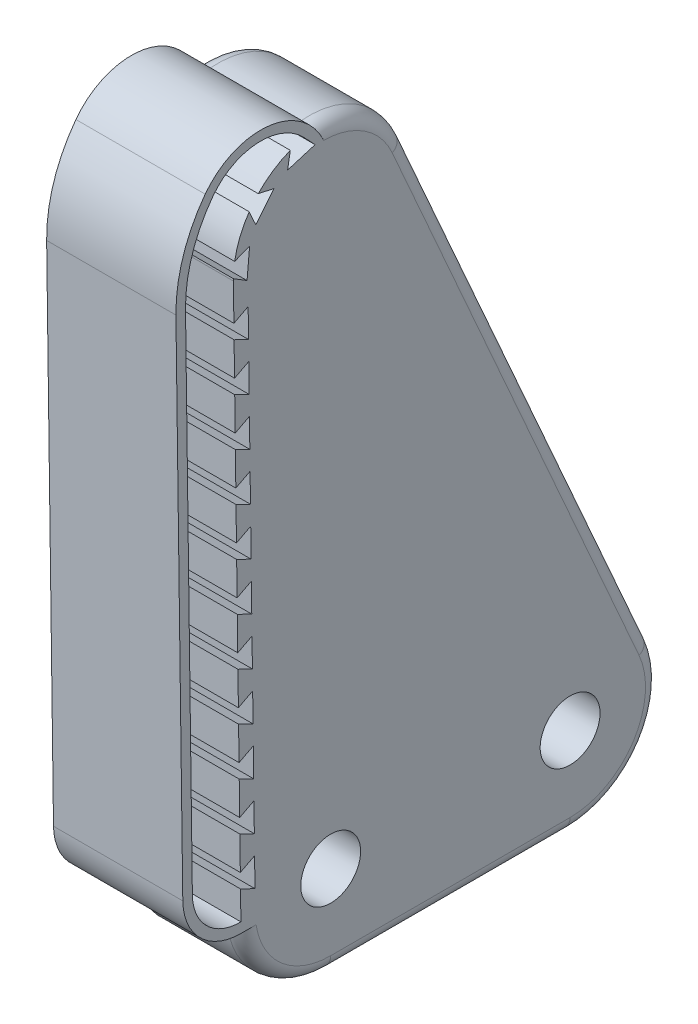
from build123d import *

# Parameters (mm, degrees)
BOSS_EXTRUDE1_DEPTH = 6.35
SKETCH2_R           = 1.5875
CUT_EXTRUDE1_DEPTH  = 38.1
CUT_EXTRUDE2_DEPTH  = 6.35
LPATTERN1_COUNT     = 11
LPATTERN1_PITCH     = 2.54
CUT_EXTRUDE3_START  = -6.35
CUT_EXTRUDE3_DEPTH  = 6.35
CIRPATTERN1_COUNT   = 3
CIRPATTERN1_ANGLE   = 68
BOSS_EXTRUDE2_DEPTH = 6.35
BOSS_EXTRUDE3_START = 0.508
BOSS_EXTRUDE3_DEPTH = 0.508
FILLET3_R           = 0.762
SCALE_RATIO_1_SCALE = 1.3


with BuildPart() as part:
    # Sketch1 → Boss-Extrude1 (new body)
    with BuildSketch(Plane(origin=(0, 0, 0), x_dir=(0, 0, -1), z_dir=(1, 0, 0))):
        with BuildLine():
            Line((0, -4.7625), (12.7, -4.7625))
            ThreePointArc((12.7, -4.7625), (16.69058737, -2.599349668), (17.05608691, 1.925074826))
            Line((17.05608691, 1.925074826), (3.957741706, 31.564198098))
            ThreePointArc((3.957741706, 31.564198098), (-1.413387908, 34.29219694), (-5.160415138, 29.575121793))
            Line((-5.160415138, 29.575121793), (-4.762069934, -0.064001479))
            ThreePointArc((-4.762069934, -0.064001479), (-3.344891568, -3.39014847), (0, -4.7625))
        make_face()
    extrude(amount=BOSS_EXTRUDE1_DEPTH)

    # Sketch2 → Cut-Extrude1 (cut)
    with BuildSketch(Plane(origin=(6.35, 0, 0), x_dir=(0, 0, -1), z_dir=(1, 0, 0))):
        Circle(SKETCH2_R)
        with Locations((12.7, 0)):
            Circle(SKETCH2_R)
    extrude(amount=-CUT_EXTRUDE1_DEPTH, mode=Mode.SUBTRACT)

    # Sketch3 → Cut-Extrude2 (cut)
    with BuildSketch(Plane(origin=(6.35, 0, 0), x_dir=(0, 0, -1), z_dir=(1, 0, 0))):
        Polygon((-4.782550408, 1.4598609), (-4.792790644, 2.22179209), (-4.035979573, 2.612997921), (-4.0154991, 1.089135542), align=None)
    cut_extrude2 = extrude(amount=-CUT_EXTRUDE2_DEPTH, mode=Mode.SUBTRACT)

    # LPattern1: Cut-Extrude2 ×11
    with Locations(*[Vector(0, 0.9999096975250266, 0.013438630711869543) * (i * LPATTERN1_PITCH) for i in range(1, LPATTERN1_COUNT)]):
        add(cut_extrude2, mode=Mode.SUBTRACT)

    # Sketch5 → Cut-Extrude3 (cut)
    with BuildSketch(Plane(origin=(6.35, 0, 0), x_dir=(0, 0, -1), z_dir=(1, 0, 0)).offset(CUT_EXTRUDE3_START)):
        with BuildLine():
            Line((-2.14250095, 34.070751301), (-2.285611832, 33.230915438))
            Line((-2.285611832, 33.230915438), (-0.827385747, 33.673806717))
            Line((-0.827385747, 33.673806717), (-1.413387908, 34.29219694))
            ThreePointArc((-1.413387908, 34.29219694), (-1.782380451, 34.196079788), (-2.14250095, 34.070751301))
        make_face()
    cut_extrude3 = extrude(amount=CUT_EXTRUDE3_DEPTH, mode=Mode.SUBTRACT)

    # CirPattern1: Cut-Extrude3 ×3 about axis
    cirpattern1_axis = Axis((0, 29.639123272, 0.398345204), (1, 0, 0))
    for i in range(1, CIRPATTERN1_COUNT):
        add(cut_extrude3.rotate(cirpattern1_axis, i * CIRPATTERN1_ANGLE / (CIRPATTERN1_COUNT - 1)), mode=Mode.SUBTRACT)

    # Sketch6 → Boss-Extrude2 (add)
    with BuildSketch(Plane(origin=(0, 0, 0), x_dir=(0, 0, -1), z_dir=(1, 0, 0))):
        with BuildLine():
            Line((-7.335974688, 2.441635031), (-7.70018577, 29.540987671))
            ThreePointArc((-7.70018577, 29.540987671), (-7.343715671, 31.89485715), (-6.249061464, 34.008977446))
            ThreePointArc((-6.249061464, 34.008977446), (-3.897096462, 35.275278165), (-1.413387908, 34.29219694))
            ThreePointArc((-1.413387908, 34.29219694), (-1.118769293, 34.346818609), (-0.821298902, 34.382805009))
            ThreePointArc((-0.821298902, 34.382805009), (-3.75592559, 35.788432355), (-6.656067812, 34.312967301))
            ThreePointArc((-6.656067812, 34.312967301), (-7.826871877, 32.051777768), (-8.208139896, 29.534160847))
            Line((-8.208139896, 29.534160847), (-7.844020566, 2.441635031))
            ThreePointArc((-7.844020566, 2.441635031), (-6.92684089, 0.288995326), (-4.762069934, -0.599172997))
            Line((-4.762069934, -0.599172997), (-4.724658503, -0.599172997))
            ThreePointArc((-4.724658503, -0.599172997), (-4.750905835, -0.332114438), (-4.762069934, -0.064001479))
            ThreePointArc((-4.762069934, -0.064001479), (-6.567956624, 0.655743647), (-7.335974688, 2.441635031))
        make_face()
    extrude(amount=BOSS_EXTRUDE2_DEPTH)

    # Sketch7 → Boss-Extrude3 (add)
    with BuildSketch(Plane.ZY.offset(BOSS_EXTRUDE3_START)):
        with BuildLine():
            Line((3.890529822, 29.592188854), (3.484762618, -0.599172997))
            Line((3.484762618, -0.599172997), (4.762069934, -0.599172997))
            ThreePointArc((4.762069934, -0.599172997), (6.92684089, 0.288995326), (7.844020566, 2.441635031))
            Line((7.844020566, 2.441635031), (8.208139896, 29.534160847))
            ThreePointArc((8.208139896, 29.534160847), (7.826871877, 32.051777768), (6.656067812, 34.312967301))
            ThreePointArc((6.656067812, 34.312967301), (3.75592559, 35.788432355), (0.821298902, 34.382805009))
            Line((0.821298902, 34.382805009), (-0.201439925, 33.079735725))
            ThreePointArc((-0.201439925, 33.079735725), (2.663789861, 32.297189628), (3.890529822, 29.592188854))
        make_face()
    extrude(amount=-BOSS_EXTRUDE3_DEPTH)

    # Fillet3
    fillet3_edges = [part.edges().sort_by_distance(p)[0] for p in [
        (6.35, -2.599349668, -16.69058737),
        (6.35, 16.744636462, -10.506914308),
        (6.35, 33.741303888, -2.021059773),
        (0, -3.573161601, 3.148638186),
        (6.35, -3.573161601, 3.148638186),
        (0, 33.741303888, -2.021059773),
        (0, 16.744636462, -10.506914308),
        (6.35, -4.7625, -6.35),
        (0, -2.599349668, -16.69058737),
        (0, -4.7625, -6.35),
    ]]
    fillet(fillet3_edges, radius=FILLET3_R)


with BuildPart() as part_1:
    # Scale ratio 1: scaled about (0, 0, 0)
    add(part.part.scale(SCALE_RATIO_1_SCALE))


solid = part_1.part
